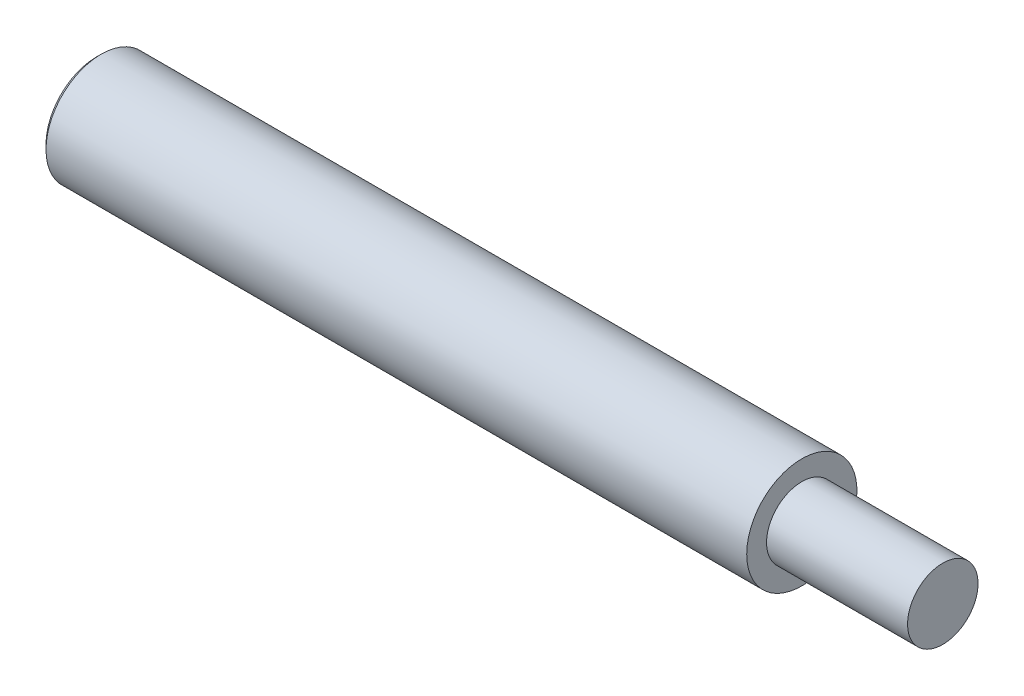
from build123d import *

# Parameters (mm, degrees)
CHAMFER1_SIZE = 1


with BuildPart() as part:
    # Sketch1 → Revolve1 (revolve)
    with BuildSketch(Plane.XY, mode=Mode.PRIVATE) as revolve1_sk:
        Polygon((0, 0), (0, 12.5), (160, 12.5), (160, 8), (192, 8), (192, 0), align=None)
    revolve(revolve1_sk.sketch.rotate(Axis((0, 0, 0), (1, 0, 0)), 90), axis=Axis((0, 0, 0), (1, 0, 0)))

    # Chamfer1
    chamfer1_edges = [part.edges().sort_by_distance(p)[0] for p in [
        (0, 0, -12.5),
    ]]
    chamfer(chamfer1_edges, length=CHAMFER1_SIZE)


solid = part.part
